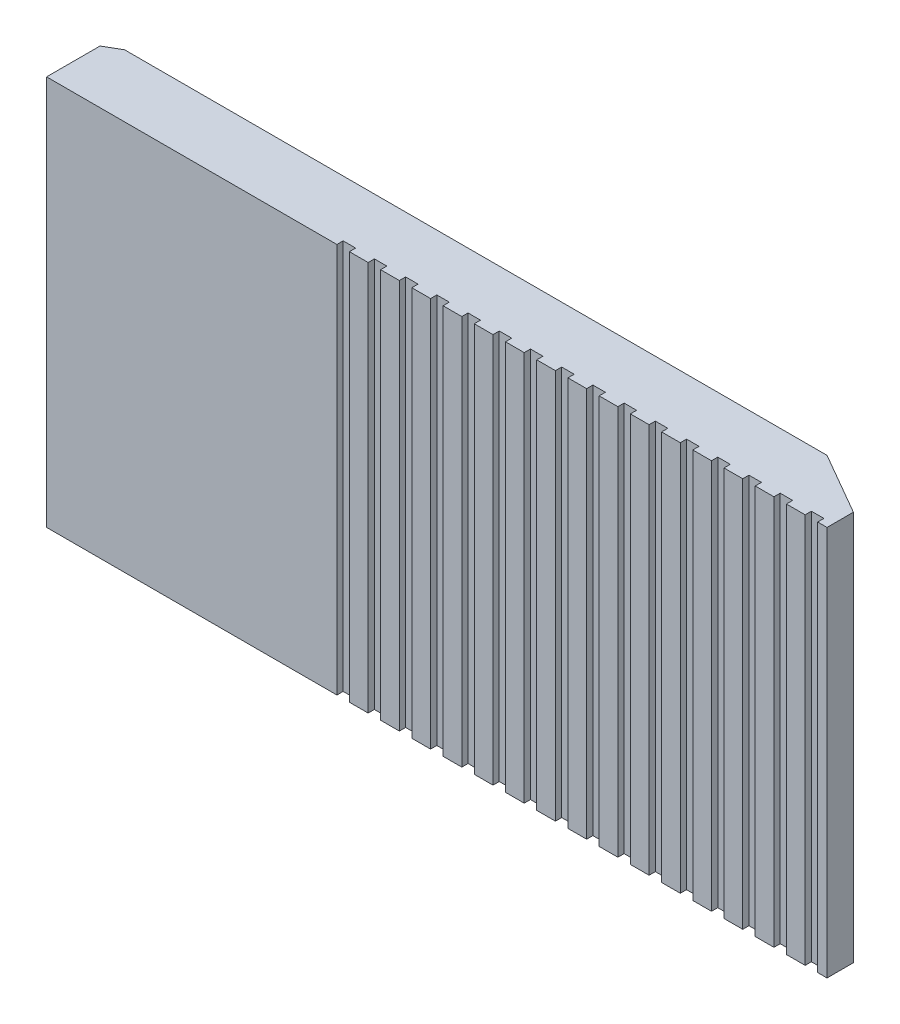
SolidWorks part; units mm, degrees
ref_plane "Front Plane" through (0, 0, 0) normal (0, 0, 1) x (1, 0, 0)
ref_plane "Top Plane" through (0, 0, 0) normal (0, 1, 0) x (1, 0, 0)
ref_plane "Right Plane" through (0, 0, 0) normal (1, 0, 0) x (0, 0, -1)
sketch "Sketch1" plane through (0, 0, 0) normal (0, 0, 1) x (1, 0, 0)
  line L1 (-25, 12.5) -> (25, 12.5)
  line L2 (-25, 12.5) -> (-25, -12.5)
  line L3 (-25, -12.5) -> (25, -12.5)
  line L4 (25, 12.5) -> (25, -12.5)
  line L5 (-25, 12.5) -> (25, -12.5) construction
  line L6 (-25, -12.5) -> (25, 12.5) construction
  point P0 (0, 0)
  dimension "D1" = 50
  dimension "D2" = 25
extrude "Boss-Extrude1" add sketch "Sketch1" along normal blind 4
chamfer "Chamfer1" distance 4 angle 30 1 edges at (25, 0, 0)
sketch "Sketch2" plane through (0, 0, 0) normal (0, 0, -1) x (-1, 0, 0)
  line L0 (-25, 0) -> (-10, 0) construction
  line L1 (-25, -12.5) -> (-25, 12.5) construction
  line L3 (-15, -5) -> (-5, -5)
  line L4 (-15, -5) -> (-15, 5)
  line L5 (-15, 5) -> (-5, 5)
  line L6 (-5, -5) -> (-5, 5)
  line L7 (-15, -5) -> (-5, 5) construction
  line L8 (-15, 5) -> (-5, -5) construction
  dimension "D1" = 10
  dimension "D2" = 15
  dimension "D3" = 10
extrude "Boss-Extrude2" add sketch "Sketch2" along normal blind 5.5
sketch "Sketch3" plane through (0, 12.5, 0) normal (0, 1, 0) x (1, 0, 0)
  line L0 (25, -4) -> (-25, -4) construction
  line L1 (23.6, -3.6) -> (24.4, -3.6)
  line L2 (23.6, -3.6) -> (23.6, -4.4)
  line L3 (23.6, -4.4) -> (24.4, -4.4)
  line L4 (24.4, -3.6) -> (24.4, -4.4)
  line L5 (23.6, -3.6) -> (24.4, -4.4) construction
  line L6 (23.6, -4.4) -> (24.4, -3.6) construction
  line L7 (25, -4) -> (25, -2.3094) construction
  point P0 (24, -4)
  dimension "D1" = 0.8
  dimension "D2" = 0.8
  dimension "D3" = 1
extrude "Cut-Extrude1" cut sketch "Sketch3" against normal through all
pattern_linear "LPattern1" count 16 spacing 2 along (-1, 0, 0) of "Cut-Extrude1"
chamfer "Chamfer2" distance 1 angle 30 1 edges at (-25, 0, 0)
